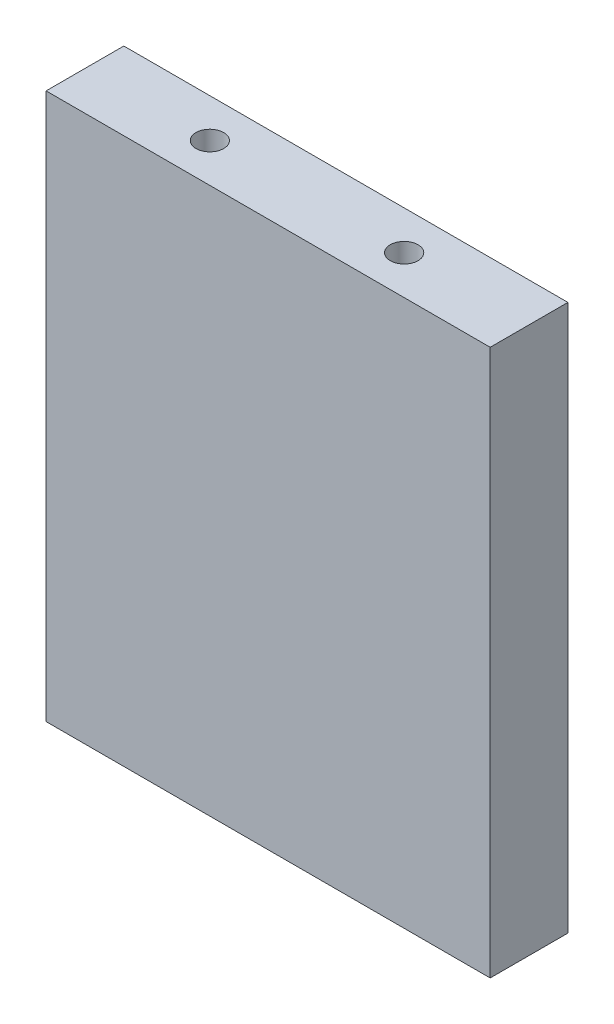
SolidWorks part; units mm, degrees
ref_plane "前视" through (0, 0, 0) normal (0, 0, 1) x (1, 0, 0)
ref_plane "上视" through (0, 0, 0) normal (0, 1, 0) x (1, 0, 0)
ref_plane "右视" through (0, 0, 0) normal (1, 0, 0) x (0, 0, -1)
sketch "草图1" plane through (0, 0, 0) normal (0, 0, 1) x (1, 0, 0)
  line L1 (-40, 49.2) -> (40, 49.2)
  line L2 (-40, 49.2) -> (-40, -49.2)
  line L3 (-40, -49.2) -> (40, -49.2)
  line L4 (40, 49.2) -> (40, -49.2)
  line L5 (-40, 49.2) -> (40, -49.2) construction
  line L6 (-40, -49.2) -> (40, 49.2) construction
  point P0 (0, 0)
  dimension "D1" = 80
  dimension "D2" = 98.4
extrude "凸台-拉伸1" add sketch "草图1" along normal blind 14
hole_wizard "M6 螺纹孔1" positions "草图3" profile "草图2" tap size "M6" standard "GB"
sketch "草图3" plane through (0, -49.2, 0) normal (0, -1, 0) x (-1, 0, 0)
  point P0 (-21, -7)
  point P3 (21, -7)
sketch "草图2" plane through (21, -49.2, 7) normal (1, 0, 0) x (0, 0, -1)
  line L0 (0, 0) -> (0, 18.5022)
  line L1 (0, 18.5022) -> (2.5, 17)
  line L2 (2.5, 17) -> (2.5, 0)
  line L5 (2.5, 0) -> (0, 0)
  line L10 (0, 18.5022) -> (-2.5, 17) construction
  line L11 (0, -6.35) -> (0, 107.95) construction
  dimension "螺纹孔钻头直径" = 5
  dimension "螺纹孔钻头深度" = 17
  dimension "导头角度" = 118
cosmetic thread "孔螺蚊线1" parameters "D1"=12, "D2"=6
cosmetic thread "孔螺蚊线2" parameters "D1"=12, "D2"=6
hole_wizard "M6 螺纹孔2" positions "草图5" profile "草图4" tap size "M6" standard "GB"
sketch "草图5" plane through (0, 49.2, 0) normal (0, 1, 0) x (1, 0, 0)
  line L0 (0, 0) -> (0, -27.2928) construction
  line L2 (-40, -7) -> (-13.716, -7) construction
  line L3 (-40, -14) -> (-40, 0) construction
  point P0 (-17.5, -7)
  point P2 (17.5, -7)
  dimension "D1" = 35
sketch "草图4" plane through (-17.5, 49.2, 7) normal (1, 0, 0) x (0, 0, 1)
  line L0 (0, 0) -> (0, 18.5022)
  line L1 (0, 18.5022) -> (2.5, 17)
  line L2 (2.5, 17) -> (2.5, 0)
  line L5 (2.5, 0) -> (0, 0)
  line L10 (0, 18.5022) -> (-2.5, 17) construction
  line L11 (0, -6.35) -> (0, 107.95) construction
  dimension "螺纹孔钻头直径" = 5
  dimension "螺纹孔钻头深度" = 17
  dimension "导头角度" = 118
cosmetic thread "孔螺蚊线3" parameters "D1"=12, "D2"=6
cosmetic thread "孔螺蚊线4" parameters "D1"=12, "D2"=6
